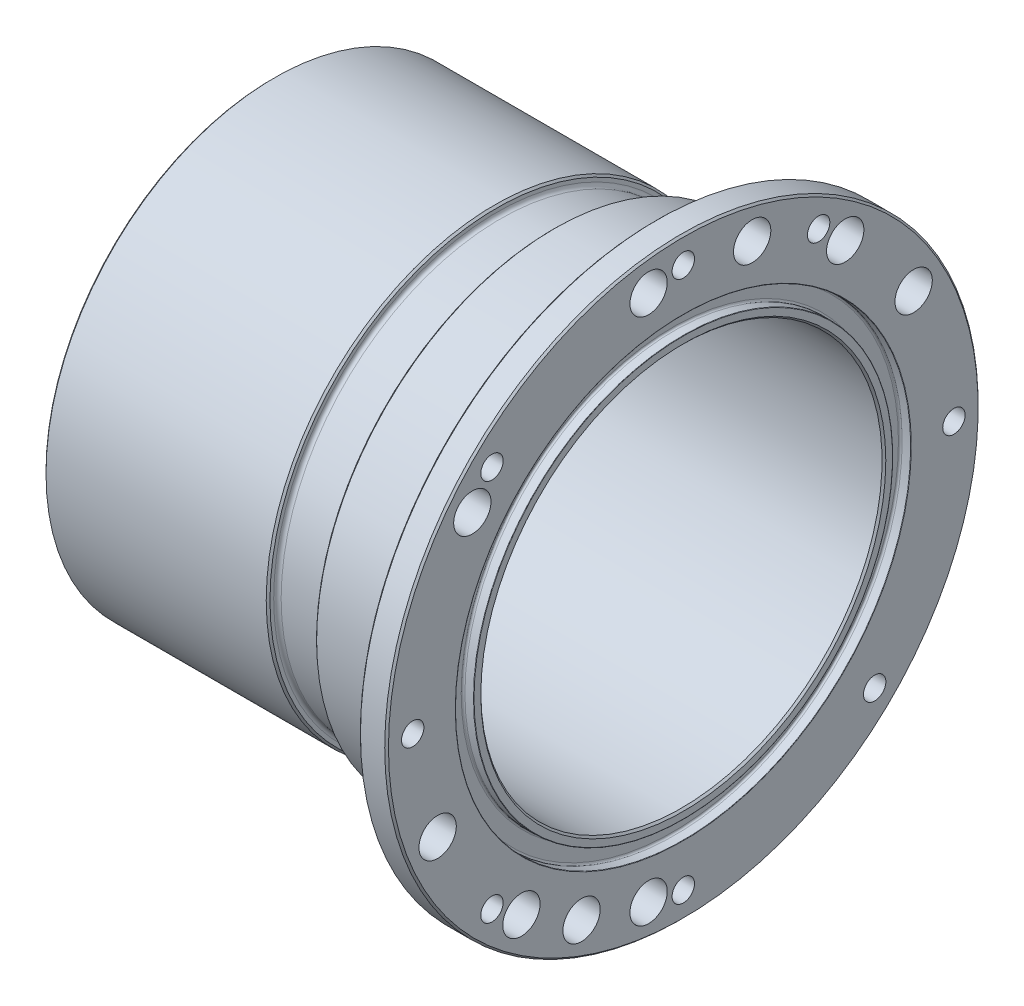
from build123d import *

# Parameters (mm, degrees)
SKETCH2_R          = 6
CUT_EXTRUDE1_DEPTH = 305.281120019
FILLET1_R          = 2
CHAMFER1_SIZE      = 1
FILLET2_R          = 2
CHAMFER2_SIZE      = 1
SKETCH4_R          = 10
CUT_EXTRUDE2_DEPTH = 305.281120019


with BuildPart() as part:
    # Sketch1 → Revolve1 (revolve)
    with BuildSketch(Plane.XY, mode=Mode.PRIVATE) as revolve1_sk:
        with BuildLine():
            Line((0, 107.5), (220, 107.5))
            Line((220, 107.5), (220, 112.1))
            ThreePointArc((220, 112.1), (219.941421356, 112.241421356), (219.8, 112.3))
            Line((219.8, 112.3), (215.28, 112.3))
            ThreePointArc((215.28, 112.3), (214.572893219, 112.592893219), (214.28, 113.3))
            Line((214.28, 113.3), (214.28, 121))
            ThreePointArc((214.28, 121), (214.572893219, 121.707106781), (215.28, 122))
            Line((215.28, 122), (219.8, 122))
            ThreePointArc((219.8, 122), (219.941421356, 122.058578644), (220, 122.2))
            Line((220, 122.2), (220, 159))
            Line((220, 159), (205, 159))
            Line((205, 159), (205, 127.5))
            Line((205, 127.5), (150, 127.5))
            Line((150, 127.5), (150, 117.5))
            Line((150, 117.5), (120, 117.5))
            Line((120, 117.5), (120, 122.5))
            Line((120, 122.5), (0, 122.5))
            Line((0, 122.5), (0, 107.5))
        make_face()
    revolve(revolve1_sk.sketch.rotate(Axis((0, 0, 0), (1, 0, 0)), 90), axis=Axis((0, 0, 0), (1, 0, 0)))

    # Sketch2 → Cut-Extrude1 (cut, through all)
    with BuildSketch(Plane.ZY.offset(-205)):
        with Locations((-72.5, 125.573683549)):
            Circle(SKETCH2_R)
        with Locations((0, 145)):
            Circle(SKETCH2_R)
        with Locations((102.530483272, 102.530483272)):
            Circle(SKETCH2_R)
        with Locations((145, 0)):
            Circle(SKETCH2_R)
        with Locations((102.530483272, -102.530483272)):
            Circle(SKETCH2_R)
        with Locations((0, -145)):
            Circle(SKETCH2_R)
        with Locations((-102.530483272, -102.530483272)):
            Circle(SKETCH2_R)
        with Locations((-145, 0)):
            Circle(SKETCH2_R)
    extrude(amount=-CUT_EXTRUDE1_DEPTH, mode=Mode.SUBTRACT)

    # Fillet1
    fillet1_edges = [part.edges().sort_by_distance(p)[0] for p in [
        (120, 0, -117.5),
        (150, 0, -117.5),
    ]]
    fillet(fillet1_edges, radius=FILLET1_R)

    # Chamfer1
    chamfer1_edges = [part.edges().sort_by_distance(p)[0] for p in [
        (0, 0, -122.5),
        (120, 0, -122.5),
        (150, 0, -127.5),
        (205, 0, -159),
        (220, 0, -159),
        (0, 0, -107.5),
    ]]
    chamfer(chamfer1_edges, length=CHAMFER1_SIZE)

    # Fillet2
    fillet2_edges = [part.edges().sort_by_distance(p)[0] for p in [
        (205, 0, -127.5),
    ]]
    fillet(fillet2_edges, radius=FILLET2_R)

    # Chamfer2
    chamfer2_edges = [part.edges().sort_by_distance(p)[0] for p in [
        (220, 0, -107.5),
    ]]
    chamfer(chamfer2_edges, length=CHAMFER2_SIZE)

    # Sketch4 → Cut-Extrude2 (cut, through all)
    with BuildSketch(Plane.ZY.offset(-205)):
        with Locations((-123.408620039, 71.25)):
            Circle(SKETCH4_R)
        with Locations((-86.748503634, 113.052850992)):
            Circle(SKETCH4_R)
        with Locations((-36.881713927, 137.644430246)):
            Circle(SKETCH4_R)
        with Locations((18.599982391, 141.280892746)):
            Circle(SKETCH4_R)
        with Locations((113.052850992, 86.748503634)):
            Circle(SKETCH4_R)
        with Locations((131.652833383, -54.532389112)):
            Circle(SKETCH4_R)
        with Locations((86.748503634, -113.052850992)):
            Circle(SKETCH4_R)
        with Locations((54.532389112, -131.652833383)):
            Circle(SKETCH4_R)
        with Locations((18.599982391, -141.280892746)):
            Circle(SKETCH4_R)
    extrude(amount=-CUT_EXTRUDE2_DEPTH, mode=Mode.SUBTRACT)


solid = part.part
